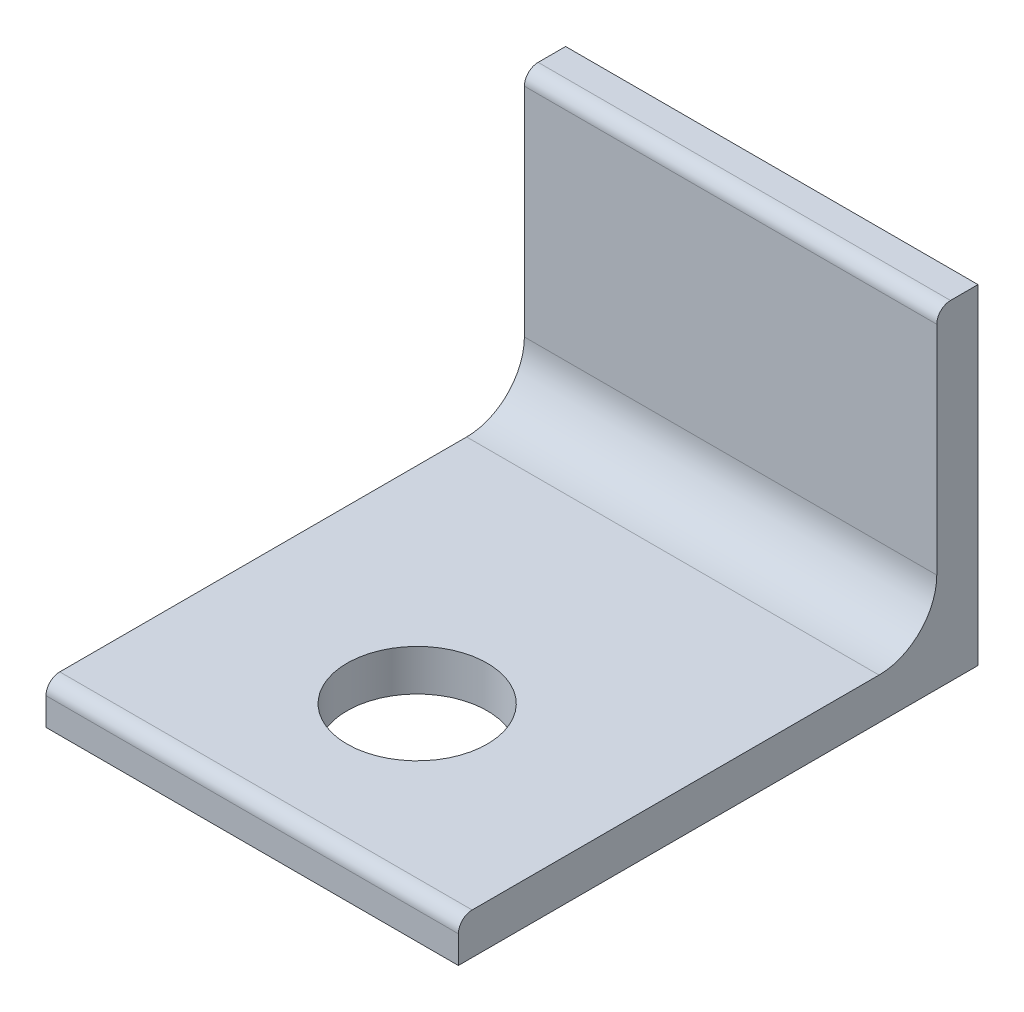
from build123d import *

# Parameters (mm, degrees)
UNEQUAL_ANGLE_6_3_4_5_1_DEPTH = 50
SKETCH3_R                     = 8.5
CUT_EXTRUDE1_DEPTH            = 10


with BuildPart() as part:
    # Sketch1 → Unequal Angle 6.3-4-5(1) (new body)
    with BuildSketch(Plane(origin=(0, 0, 0), x_dir=(0, 0, 1), z_dir=(1, 0, 0))):
        with BuildLine():
            Line((63, 0), (0, 0))
            Line((0, 0), (0, -40))
            Line((0, -40), (3.333333333, -40))
            ThreePointArc((3.333333333, -40), (4.511844635, -39.511844635), (5, -38.333333333))
            Line((5, -38.333333333), (5, -12))
            ThreePointArc((5, -12), (7.050252532, -7.050252532), (12, -5))
            Line((12, -5), (61.333333333, -5))
            ThreePointArc((61.333333333, -5), (62.511844635, -4.511844635), (63, -3.333333333))
            Line((63, -3.333333333), (63, 0))
        make_face()
    extrude(amount=UNEQUAL_ANGLE_6_3_4_5_1_DEPTH)

    # Sketch3 → Cut-Extrude1 (cut)
    with BuildSketch(Plane(origin=(0, 5, 0), x_dir=(1, 0, 0), z_dir=(0, 1, 0))):
        with Locations(Location((25, -43, 0), (0, 0, 270))):
            Circle(SKETCH3_R)
    extrude(amount=-CUT_EXTRUDE1_DEPTH, mode=Mode.SUBTRACT)


solid = part.part
